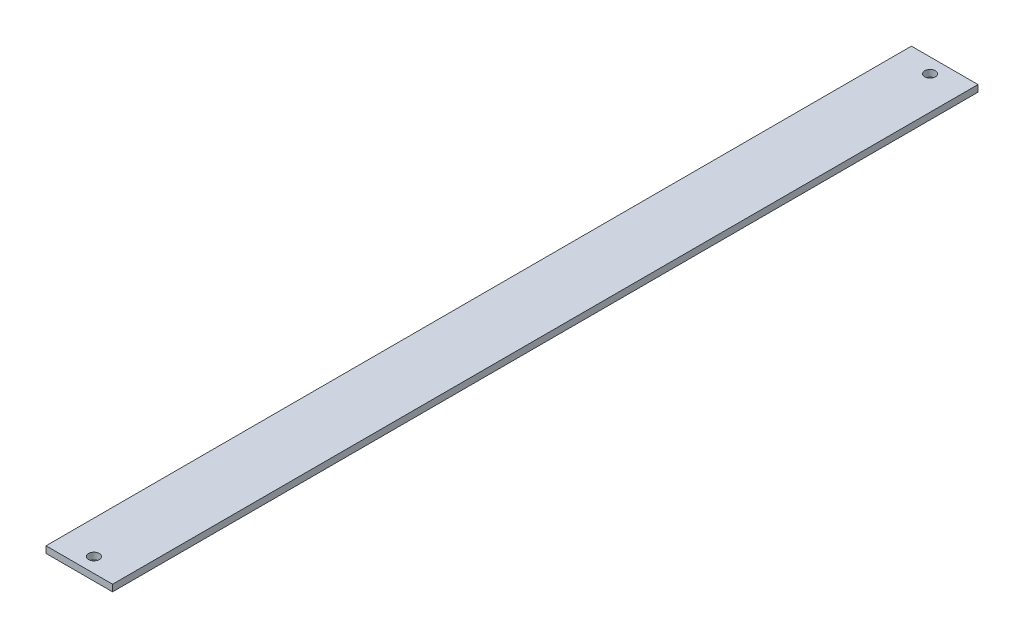
from build123d import *

# Parameters (mm, degrees)
SKETCH_1_W          = 50
SKETCH_1_H          = 650
EXTRUDE_1_DEPTH     = 5
SKETCH_2_R          = 4
CUT_EXTRUDE_1_DEPTH = 326.998466254


with BuildPart() as part:
    # 草图1 → 凸台-拉伸1 (new body)
    with BuildSketch(Plane(origin=(0, 0, 0), x_dir=(1, 0, 0), z_dir=(0, 1, 0))):
        Rectangle(SKETCH_1_W, SKETCH_1_H)
    extrude(amount=EXTRUDE_1_DEPTH)

    # 草图2 → 切除-拉伸1 (cut, through all)
    with BuildSketch(Plane(origin=(0, 5, 0), x_dir=(1, 0, 0), z_dir=(0, 1, 0))):
        with Locations(Location((0, 314, 0), (0, 0, 270))):
            Circle(SKETCH_2_R)
        with Locations(Location((0, -314, 0), (0, 0, 90))):
            Circle(SKETCH_2_R)
    extrude(amount=-CUT_EXTRUDE_1_DEPTH, mode=Mode.SUBTRACT)


solid = part.part
